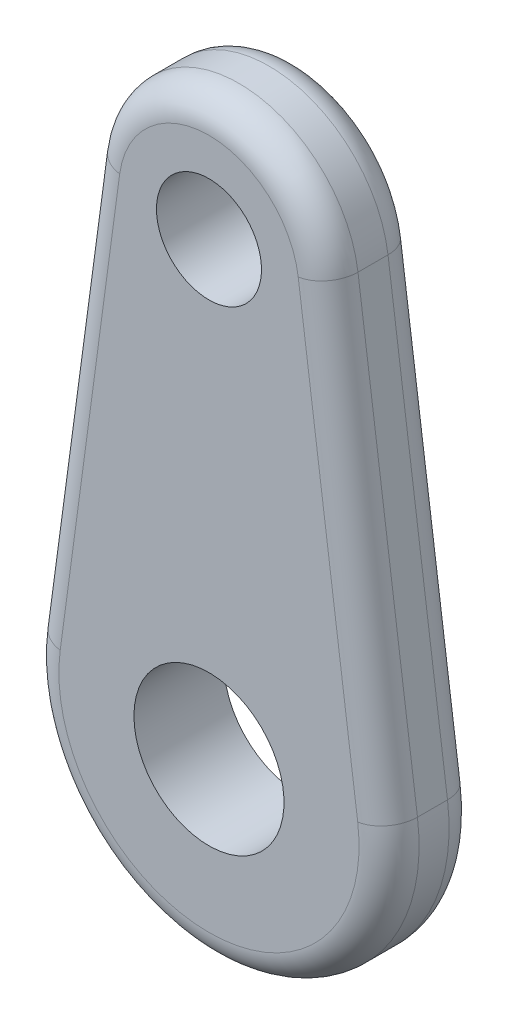
SolidWorks part; units mm, degrees
ref_plane "Front Plane" through (0, 0, 0) normal (0, 0, 1) x (1, 0, 0)
ref_plane "Top Plane" through (0, 0, 0) normal (0, 1, 0) x (1, 0, 0)
ref_plane "Right Plane" through (0, 0, 0) normal (1, 0, 0) x (0, 0, -1)
ref_plane "Plane1" through (0, 0, 30) normal (0, 0, 1) x (1, 0, 0)
sketch "Sketch1" plane through (0, 0, 30) normal (0, 0, 1) x (1, 0, 0)
  line L0 (59.4643, 8) -> (39.6428, 155.3333)
  line L1 (-39.6428, 155.3333) -> (-59.4643, 8)
  arc A0 (-59.4643, 8) -> (59.4643, 8) centre (0, 0) ccw
  arc A1 (39.6428, 155.3333) -> (-39.6428, 155.3333) centre (0, 150) ccw
extrude "Boss-Extrude1" add sketch "Sketch1" against normal blind 30
hole_wizard "M30 Clearance Hole1" positions "Sketch3" profile "Sketch2" hole size "M30" standard "ANSI Metric"
sketch "Sketch3" plane through (0, 0, 0) normal (0, 0, -1) x (-1, 0, 0)
  point P0 (0, 150)
sketch "Sketch2" plane through (0, 150, 0) normal (1, 0, 0) x (0, 1, 0)
  line L0 (0, 0) -> (0, 30)
  line L1 (0, 30) -> (17.5, 30)
  line L2 (17.5, 30) -> (17.5, 0)
  line L5 (17.5, 0) -> (0, 0)
  line L11 (0, -6.35) -> (0, 107.95) construction
  dimension "通孔孔直径" = 35
  dimension "通孔孔深度" = 30
hole_wizard "M45 Clearance Hole1" positions "Sketch5" profile "Sketch4" hole size "M45" standard "ANSI Metric"
sketch "Sketch5" plane through (0, 0, 0) normal (0, 0, -1) x (-1, 0, 0)
  point P0 (0, 0)
sketch "Sketch4" plane through (0, 0, 0) normal (1, 0, 0) x (0, 1, 0)
  line L0 (0, 0) -> (0, 30)
  line L1 (0, 30) -> (25, 30)
  line L2 (25, 30) -> (25, 0)
  line L5 (25, 0) -> (0, 0)
  line L11 (0, -6.35) -> (0, 107.95) construction
  dimension "通孔孔直径" = 50
  dimension "通孔孔深度" = 30
fillet "Fillet1" radius 10 8 edges at (0, 190, 30) (49.5536, 81.6667, 30) (-49.5536, 81.6667, 30) (0, -60, 30) (49.5536, 81.6667, 0) (0, -60, 0) (0, 190, 0) (-49.5536, 81.6667, 0)
